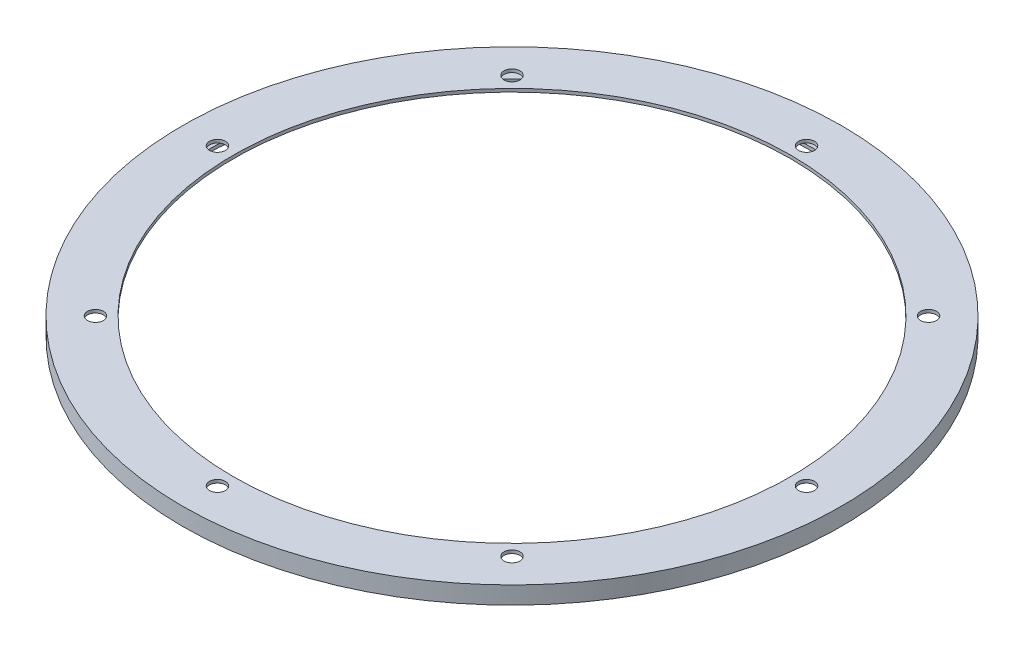
SolidWorks part; units mm, degrees
ref_plane "Front Plane" through (0, 0, 0) normal (0, 0, 1) x (1, 0, 0)
ref_plane "Top Plane" through (0, 0, 0) normal (0, 1, 0) x (1, 0, 0)
ref_plane "Right Plane" through (0, 0, 0) normal (1, 0, 0) x (0, 0, -1)
other "Configuration Table"
sketch "Sketch1" plane through (0, 0, 0) normal (0, 1, 0) x (1, 0, 0)
  circle A0 centre (0, 0) radius 205
  circle A1 centre (-185, 0) radius 5
  circle A2 centre (0, 0) radius 175
  circle A3 centre (-130.8148, 130.8148) radius 5
  circle A4 centre (0, 185) radius 5
  circle A5 centre (130.8148, 130.8148) radius 5
  circle A6 centre (185, 0) radius 5
  circle A7 centre (130.8148, -130.8148) radius 5
  circle A8 centre (0, -185) radius 5
  circle A9 centre (-130.8148, -130.8148) radius 5
  point P23 (0, 0)
  dimension "D1" = 410
  dimension "D2" = 10
  dimension "D3" = 185
  dimension "D4" = 30
  dimension "D5" = 8
extrude "Boss-Extrude1" add sketch "Sketch1" along normal blind 2
sketch "Sketch2" plane through (0, 0, 0) normal (0, -1, 0) x (1, 0, 0)
  circle A0 centre (0, 0) radius 207
  circle A1 centre (0, 0) radius 205
extrude "Boss-Extrude2" add sketch "Sketch2" along normal blind 7 and the other way blind 2
sketch "Sketch3" plane through (0, -7, 0) normal (0, -1, 0) x (1, 0, 0)
  circle A0 centre (0, 0) radius 207
  circle A1 centre (0, 0) radius 195
extrude "Boss-Extrude3" add sketch "Sketch3" along normal blind 2
